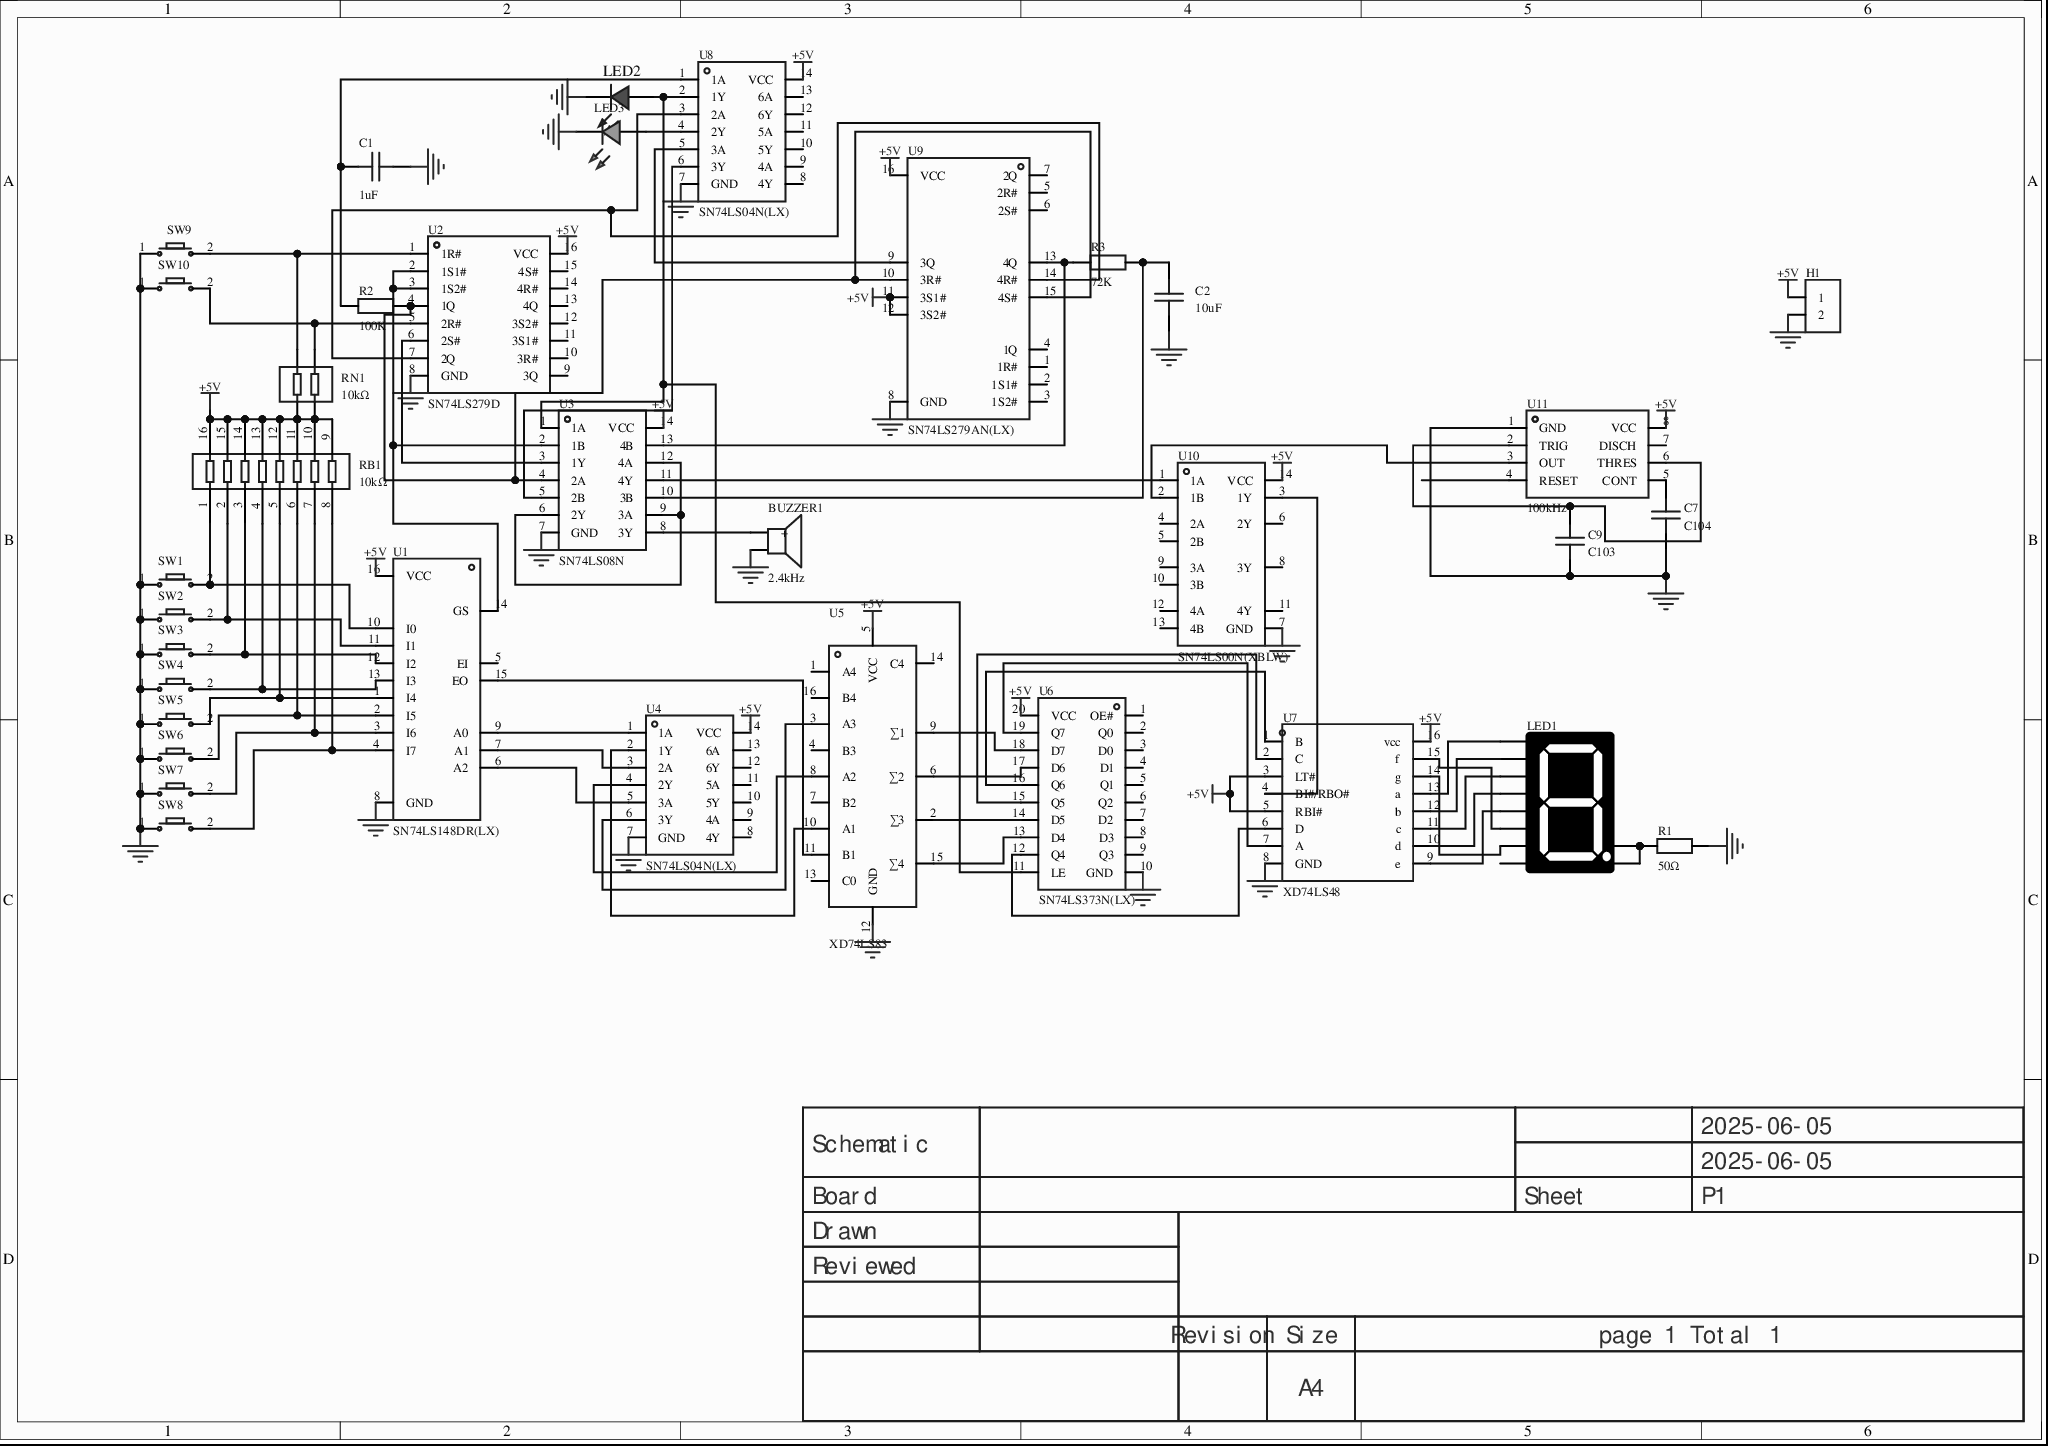
[diagram p0: MISC51700-3.schdoc]
# Altium project MISC51700-2.PrjPcb
1 sheet, 35 parts. Net scope: global (net labels, ports and power ports of the same name join across sheets).
Board file: MISC51700.pcbdoc

## Sheet MISC51700-3.schdoc
size 297 x 209 mm; Version: V1.0; @Project Name: MISC51700; @Page Count: 1; @Update Date: 2025-06-05; @Create Date: 2025-06-05; @Schematic Name: MISC51700; @Page No: 1; @Create Time: 06:48:36; @Update Time: 17:09:20; @Board Name: MISC51700

### Parts
BUZZER1  2.4kHz  [BUZ-TH_BD12.0-P7.60-D0.6-FD]
C1  1uF  [C0603]
C2  10uF  [C0603]
C7  C104  [CAP-TH_L8.5-W5.0-P5.00-D1.2]
C9  C103  [CAP-TH_L8.5-W5.0-P5.00-D1.2]
H1  (no value)  [HDR-TH_2P-P2.54-V-F]
LED1  (no value)  [LED-SEG-TH_10P-L12.6-W19.0-P2.54-S15.24-BL]
LED2  (no value)  [LED_0805]
LED3  (no value)  [LED_0805]
R1  50Ω  [R0603]
R2  100K  [R0805]
R3  72K  [R0805]
RB1  10kΩ  [RES-ARRAY-SMD_0603-16P-L6.4-W1.6-TL]
RN1  10kΩ  [RES-ARRAY-SMD_0603-4P-L1.6-W1.6-BL]
SW1  (no value)  [Key_SMD_3x4x2]
SW2  (no value)  [Key_SMD_3x4x2]
SW3  (no value)  [Key_SMD_3x4x2]
SW4  (no value)  [Key_SMD_3x4x2]
SW5  (no value)  [Key_SMD_3x4x2]
SW6  (no value)  [Key_SMD_3x4x2]
SW7  (no value)  [Key_SMD_3x4x2]
SW8  (no value)  [Key_SMD_3x4x2]
SW9  (no value)  [Key_SMD_3x4x2]
SW10  (no value)  [Key_SMD_3x4x2]
U1  SN74LS148DR(LX)  [SOIC-16_L9.9-W3.9-P1.27-LS6.0-BL-1]
U2  SN74LS279D  [SOIC-16_L9.9-W3.9-P1.27-LS6.0-BL]
U3  SN74LS08N  [PDIP-14_L19.3-W6.4-P2.54-LS7.9-BL-1]
U4  SN74LS04N(LX)  [DIP-14_L19.1-W6.4-P2.54-LS7.6-BL]
U5  XD74LS83  [PDIP-16_L19.1-W6.4-P2.54-LS7.62-BL]
U6  SN74LS373N(LX)  [PDIP-20_L26.2-W7.6-P2.54-LS7.9-BL]
U7  XD74LS48  [DIP-16_L19.3-W6.4-P2.54-LS7.6-BL]
U8  SN74LS04N(LX)  [DIP-14_L19.1-W6.4-P2.54-LS7.6-BL]
U9  SN74LS279AN(LX)  [PDIP-16_L19.3-W6.4-P2.54-LS7.94-BL]
U10  SN74LS00N(XBLW)  [PDIP-14_L19.3-W6.4-P2.54-LS7.6-BL]
U11  100kHz  [DIP-8_L9.8-W6.6-P2.54-LS7.6-BL]

### Nets
+5V: H1.1 RB1.9 RB1.10 RB1.11 RB1.12 RB1.13 RB1.14 RB1.15 RB1.16 RN1.1 RN1.2 U1.16(VCC) U2.16(VCC) U3.14(VCC) U4.14(VCC) U5.5(VCC) U6.20(VCC) U7.3(LT#) U7.5(RBI#) U7.16(vcc) U8.14(VCC) U9.11(3S1#) U9.12(3S2#) U9.16(VCC) U10.14(VCC) U11.8(VCC)
GND: BUZZER1.2 C1.2 C2.1 C7.1 C9.1 H1.2 LED2.1(C) LED3.1(C) R1.1 SW1.1 SW2.1 SW3.1 SW4.1 SW5.1 SW6.1 SW7.1 SW8.1 SW9.1 SW10.1 U1.8(GND) U2.8(GND) U3.7(GND) U4.7(GND) U5.12(GND) U6.10(GND) U7.8(GND) U8.7(GND) U9.8(GND) U10.7(GND) U11.1(GND)
NetBUZZER1_1: BUZZER1.1(+) U3.8(3Y)
NetC1_1: C1.1 R2.1 U8.1(1A)
NetC2_2: C2.2 R3.2 U3.10(3B)
NetC7_2: C7.2 U11.5(CONT)
NetC9_2: C9.2 U11.2(TRIG) U11.6(THRES)
NetLED1_1: LED1.1(E) U7.9(e)
NetLED1_2: LED1.2(D) U7.10(d)
NetLED1_3: LED1.3(G1) LED1.8(G2) R1.2
NetLED1_4: LED1.4(C) U7.11(c)
NetLED1_6: LED1.6(B) U7.12(b)
NetLED1_7: LED1.7(A) U7.13(a)
NetLED1_9: LED1.9(F) U7.15(f)
NetLED1_10: LED1.10(G) U7.14(g)
NetLED2_2: LED2.2(A) U3.1(1A) U6.11(LE) U8.2(1Y)
NetLED3_2: LED3.2(A) U8.4(2Y)
NetR2_2: R2.2 U2.4(1Q) U3.4(2A) U9.10(3R#) U9.15(4S#)
NetR3_1: R3.1 U3.13(4B) U9.13(4Q)
NetRB1_1: RB1.1 SW1.2 U1.10(I0)
NetRB1_2: RB1.2 SW2.2 U1.11(I1)
NetRB1_3: RB1.3 SW3.2 U1.12(I2)
NetRB1_4: RB1.4 SW4.2 U1.13(I3)
NetRB1_5: RB1.5 SW5.2 U1.1(I4)
NetRB1_6: RB1.6 SW6.2 U1.2(I5)
NetRB1_7: RB1.7 SW7.2 U1.3(I6)
NetRB1_8: RB1.8 SW8.2 U1.4(I7)
NetRN1_3: RN1.3 SW10.2 U2.5(2R#)
NetRN1_4: RN1.4 SW9.2 U2.1(1R#)
NetU1_6: U1.6(A2) U4.5(3A)
NetU1_7: U1.7(A1) U4.3(2A)
NetU1_9: U1.9(A0) U4.1(1A)
NetU1_14: U1.14(GS) U2.2(1S1#) U2.3(1S2#) U3.2(1B)
NetU1_15: U1.15(EO) U5.11(B1)
NetU2_6: U2.6(2S#) U3.3(1Y)
NetU2_7: U2.7(2Q) U8.3(2A) U9.14(4R#)
NetU3_5: U3.5(2B) U8.6(3Y)
NetU3_6: U3.6(2Y) U3.9(3A) U3.12(4A)
NetU3_11: U3.11(4Y) U10.1(1A)
NetU4_2: U4.2(1Y) U5.10(A1)
NetU4_4: U4.4(2Y) U5.8(A2)
NetU4_6: U4.6(3Y) U5.3(A3)
NetU5_2: U5.2(∑3) U6.14(D5)
NetU5_6: U5.6(∑2) U6.17(D6)
NetU5_9: U5.9(∑1) U6.18(D7)
NetU5_15: U5.15(∑4) U6.13(D4)
NetU6_12: U6.12(Q4) U7.6(D)
NetU6_15: U6.15(Q5) U7.2(C)
NetU6_16: U6.16(Q6) U7.1(B)
NetU6_19: U6.19(Q7) U7.7(A)
NetU7_4: U7.4(BI#/RBO#) U10.3(1Y)
NetU8_5: U8.5(3A) U9.9(3Q)
NetU10_2: U10.2(1B) U11.3(OUT)

Not connected (* = marked no-connect by the designer): LED1 5(DP); U1 5(EI); U2 9(3Q) 10(3R#) 11(3S1#) 12(3S2#) 13(4Q) 14(4R#) 15(4S#); U4 8(4Y) 9(4A) 10(5Y) 11(5A) 12(6Y) 13(6A); U5 1(A4) 4(B3) 7(B2) 13(C0) 14(C4) 16(B4); U6 1(OE#) 2(Q0) 3(D0) 4(D1) 5(Q1) 6(Q2) 7(D2) 8(D3) 9(Q3); U8 8(4Y) 9(4A) 10(5Y) 11(5A) 12(6Y) 13(6A); U9 1(1R#) 2(1S1#) 3(1S2#) 4(1Q) 5(2R#) 6(2S#) 7(2Q); U10 4(2A) 5(2B) 6(2Y) 8(3Y) 9(3A) 10(3B) 11(4Y) 12(4A) 13(4B); U11 4(RESET) 7(DISCH)

### Notes on the sheet
- 2025-06-05
- Schematic
- Board
- Sheet
- P1
- Drawn
- Reviewed
- Revision
- Size
- A4
- page 1 Total 1

### Library data of the parts
BUZZER1 = TMB12A05_C96093: Drive mode:Active (built-in driver); Construction:Electromagnetic; Rated voltage:-; Frequency:2.4kHz; Sound pressure (SPL):85dB;; Manufacturer: 华能; AddInBom: yes; ModelId: 16ab50e14c5b4f2c986c135bdba60e37; ModelName: BUZ-TH_D12.0-H9.5-P7.60; ModelTransform: 472.44,472.176,0,90,0,0,-0.787,0,-177.165; Voltage - Supply: 4V~8V; Sound Pressure Level(SPL): 85dB; Symbol: TMB12A05; Device: TMB12A05_C96093; LCSC Part Name: TMB12A05; SupplierPart: C96093; ManufacturerPart: TMB12A05; Supplier Footprint: 插件,D=12mm; JLCPCB Part Class: Extended library; Datasheet: https://example.com/upload/public/pdf/source/20241025/8A17FE04D767D19A35A06DEF9A82AB1E.pdf; Supplier: LCSC; ConvertToPcb: yes; FootprintName: BUZ-TH_BD12.0-P7.60-D0.6-FD; Driver Circuitry: Active (built-in driver); Technology: Electromagnetic; Voltage Rating: -; Value: 2.4kHz; Current Consumption: -; Diameter(φD): 12mm; Length: -; Width: -; Height: 9.8mm; Operating Temperature: -
C1 C2 = CAP_0603: ConvertToPcb: yes; SymbolName: CapAcitance; ModelId: ac125912035d415993ca9572d50418b1; ModelName: C0603_L1.6-W0.8-H0.8; ModelTransform: 62.992,31.496,0,0,0,0,0,0,0; Device: CAP_0603; AddInBom: yes; Supplier Footprint: 0603; FootprintName: C0603
  C1: Value: 1uF
  C2: Value: 10uF
C7 C9 = CT4-0805B104K500F3: Capacitance:100nF; Tolerance:±10%; Rated voltage:50V; Temp coefficient:X7R;; Manufacturer: FH(风华); AddInBom: yes; ModelId: 5610b656e7164072960d9d2d8c7d4fdf; ModelName: CAP-TH_L4.2-W3.8-H3.8-P5.08; ModelTransform: 222.8342,149.606,0,0,0,0,0,0,-118.11; Tolerance: ±10%; Voltage Rated: 50V; Temperature Coefficient: X7R; Symbol: CT4-0805B104K500F3; Device: CT4-0805B104K500F3; LCSC Part Name: 100nF ±10% 50V C3型（直脚）; ManufacturerPart: CT4-0805B104K500F3; Supplier Footprint: 插件,P=5.08mm; JLCPCB Part Class: Extended library; Datasheet: https://example.com/upload/public/pdf/source/20190402/C385200_059806A6312B28FF1421A2413EB641E1.pdf; Supplier: LCSC; ConvertToPcb: yes; FootprintName: CAP-TH_L8.5-W5.0-P5.00-D1.2
  C7: Value: C104
  C9: Value: C103
H1 = HDR-F_2.54_1x2P: Symbol: Header-Female-2.54_1x2; ConvertToPcb: yes; ModelId: a9450ef445564560a104363b9aacde4e; ModelName: HDR-TH_2P-P2.54-F-LI-1X2P; ModelTransform: 215.7476,98.425,0,0,0,0,0,0,-129.921; Device: HDR-F_2.54_1x2P; AddInBom: yes; SupplierPart: C49661; Supplier Footprint: 插件; FootprintName: HDR-TH_2P-P2.54-V-F
LED1 = LED_SEG_TH_0.56x1: Symbol: LED_SEG_TH_0.56*1; ConvertToPcb: yes; ModelId: 16c3aae6d39e4ecc9e744d6eeac8d57b; ModelName: LED-SEG-TH_0.56_1p; ModelTransform: 496.062,748.03,0,0,0,0,0,0,-137.795; Device: LED_SEG_TH_0.56x1; AddInBom: yes; Supplier Footprint: 插件; FootprintName: LED-SEG-TH_10P-L12.6-W19.0-P2.54-S15.24-BL
LED2 = LED_0805-R: Symbol: LED_R; Convert to PCB: yes; 3D Model: 33fb9fca58e84f37a403ebeef4c28b77; 3D Model Transform: 78.7,49.1,39.3,0,0,0,0,0,0; ModelName: LED-0805_R; Device: LED_0805-R; Add into BOM: yes; Supplier Footprint: 0805; FootprintName: LED_0805
LED3 = LED_0805-G: Symbol: LED_G; Convert to PCB: yes; 3D Model: 381ae4d721d6485eaad9d0ca067812b5; 3D Model Transform: 63.9,39.8,31.9,0,0,0,0,0,0; ModelName: LED-0805_G; Device: LED_0805-G; Add into BOM: yes; Supplier Footprint: 0805; FootprintName: LED_0805
R1 = Res_0603: ConvertToPcb: yes; SymbolName: Resistor; ModelId: fc143cca1e79419f9cd78b61e9279f08; ModelTransform: 31.8897,63.7794,0,90,0,0,0,0,0; Value: 50Ω; Device: Res_0603; AddInBom: yes; Supplier Footprint: 0603; FootprintName: R0603; ModelName: R0603
R2 R3 = Res_0805: ConvertToPcb: yes; SymbolName: Resistor; ModelId: 37a81e68749a4138bd2dfa6897b24b85; ModelName: R0805_L2.0-W1.3-H0.6; ModelTransform: 78.74,51.181,0,0,0,0,0,-0.0005,0; Device: Res_0805; AddInBom: yes; Supplier Footprint: 0805; FootprintName: R0805
  R2: Value: 100K
  R3: Value: 72K
RB1 = 742C163103JP: Resistor count:8; Resistance:10kΩ; Tolerance:±5%; Power per element:63mW; Temp coefficient:±200ppm/℃;; Manufacturer: CTS(西迪斯); AddInBom: yes; ModelId: 221f6fb4f2034148a9d47d497d859194; ModelTransform: 251.968,64.961,0,0,0,0,0,0,0; Number of Resistors: 8; Tolerance: ±5%; Power(Watts): 63mW; Symbol: 742C163103JP; Device: 742C163103JP; LCSC Part Name: 10kΩ ±5%; SupplierPart: C2654035; ManufacturerPart: 742C163103JP; Supplier Footprint: 0603x8; JLCPCB Part Class: Extended library; Datasheet: https://example.com/upload/public/pdf/source/20210503/EA698ADAEE513162139F7667D383C0D0.pdf; Supplier: LCSC; ConvertToPcb: yes; FootprintName: RES-ARRAY-SMD_0603-16P-L6.4-W1.6-TL; ModelName: RES-ARRAY-SMD_0603-16P-L6.4-W1.6-TL; Value: 10kΩ; Temperature Coefficient: ±200ppm/℃; Number of Pins: 16
RN1 = 2D03WGJ0103T5E: Resistor count:2; Resistance:10kΩ; Tolerance:±5%; Power per element:62.5mW; Temp coefficient:±200ppm/℃;; Manufacturer: UNI-ROYAL(厚声); AddInBom: yes; ModelId: c28f3269927844d1bae4b585f2f82e94; ModelName: RES-ARRAY-SMD_0603-4P-L1.6-W1.6-H0.5-BL; ModelTransform: 62.992,62.992,0,0,0,0,0,0,0; Number of Resistors: 2; Tolerance: ±5%; Power(Watts): 62.5mW; Symbol: 2D03WGJ0103T5E; Device: 2D03WGJ0103T5E; LCSC Part Name: 10kΩ ±5%; SupplierPart: C2765531; ManufacturerPart: 2D03WGJ0103T5E; Supplier Footprint: 0603x2; JLCPCB Part Class: Extended library; Datasheet: https://example.com/upload/public/pdf/source/20210330/C2758625_90D19EEA9B8C23AA9BAF71D52BD1DB3E.pdf; Supplier: LCSC; ConvertToPcb: yes; FootprintName: RES-ARRAY-SMD_0603-4P-L1.6-W1.6-BL; Value: 10kΩ; Temperature Coefficient: ±200ppm/℃; Number of Pins: 4
SW1-SW10 = Key_SMD_3x4x2: ConvertToPcb: yes; SymbolName: Tactile switch x2; ModelId: 63599cce708d48afbce1b0db003544770819f05c4eef4c71ace90d822a990e87; ModelName: SW-SMD_L4.0-W2.9-H2-LS5.0; ModelTransform: 196.85,114.17,79.13,0,0,0,0,0,0; Device: Key_SMD_3x4x2; AddInBom: yes; Supplier Footprint: SMD; FootprintName: Key_SMD_3x4x2
U1 = SN74LS148DR(LX): Manufacturer: LX(灵星芯微); AddInBom: yes; ModelId: 19d62df4453549be81db7b702f301941; ModelName: SOIC-16_L9.9-W3.9-H1.8-LS6.0-P1.27; ModelTransform: 389.763,236.454,0,0,0,0,0,0,0; Symbol: SN74LS148DR(LX); Device: SN74LS148DR(LX); LCSC Part Name: SN74LS148DR(LX); SupplierPart: C32710673; ManufacturerPart: SN74LS148DR(LX); Supplier Footprint: SOP-16; JLCPCB Part Class: Extended library; Datasheet: https://example.com/upload/public/pdf/source/20240417/102B6FDCFA309F0B30F1058715E63CF7.pdf; Supplier: LCSC; ConvertToPcb: yes; FootprintName: SOIC-16_L9.9-W3.9-P1.27-LS6.0-BL-1
U2 = SN74LS279D: Manufacturer: onsemi(安森美); AddInBom: yes; ModelId: c21ec766ec2643efb3352f8441994f4e; ModelName: SOIC-16_L9.9-W3.9-H1.8-LS6.0-P1.27; ModelTransform: 389.763,236.454,0,0,0,0,0,0,0; Symbol: SN74LS279D; Device: SN74LS279D; LCSC Part Name: SN74LS279D; SupplierPart: C3826626; ManufacturerPart: SN74LS279D; Supplier Footprint: -; JLCPCB Part Class: Extended library; Datasheet: https://example.com/upload/public/pdf/source/20230915/97FED84B533BE8D9150AD31DF08D2AAB.pdf; Supplier: LCSC; ConvertToPcb: yes; FootprintName: SOIC-16_L9.9-W3.9-P1.27-LS6.0-BL
U3 = SN74LS08N: Logic type:AND gate; Channels:4; Operating voltage:4.75V~5.25V; Propagation delay (tpd):-;; Manufacturer: TI(德州仪器); AddInBom: yes; ModelId: 850da569defe42bfb44bffbf61585822; ModelTransform: 751.967,309.842,0,0,0,0,0,0,-118.11; Number of Channels: 4; Current - Output Low(IOL): 8mA; Current - Output High(IOH): 400uA; Input Logic Level - High: 2V; Input Logic Level - Low: 800mV; Symbol: SN74LS08N; Device: SN74LS08N; LCSC Part Name: SN74LS08N; SupplierPart: C2869595; ManufacturerPart: SN74LS08N; Supplier Footprint: PDIP-14; JLCPCB Part Class: Extended library; Supplier: LCSC; ConvertToPcb: yes; FootprintName: PDIP-14_L19.3-W6.4-P2.54-LS7.9-BL-1; ModelName: PDIP-14_L19.3-W6.4-P2.54-LS7.9-BL-1; Logic Type: AND gate; Voltage - Supply: 4.75V~5.25V; Series: 74LS series; Propagation Delay: -; Operating Temperature: 0℃~+70℃
U4 U8 = SN74LS04N(LX): Operating voltage:2V~6V; Operating current:2uA; Channels:6; Propagation delay (tpd):14ns@6V;; Manufacturer: LX(灵星芯微); AddInBom: yes; ModelId: 4fb82330961949e587245d1f3ebad69c; ModelTransform: 751.967,324.8025,0,0,0,0,0,0,-118.11; Voltage - Supply: 2V~6V; Current - Supply: 2uA; Number of Circuits: 6; Current - Output Low(IOL): 5.2mA; Input Logic Level - High: 1.5V~4.2V; Input Logic Level -Low: 500mV~1.8V; Output Logic Level - Low: 100mV~260mV; Symbol: SN74LS04N(LX); Device: SN74LS04N(LX); LCSC Part Name: SN74LS04N(LX); SupplierPart: C22374093; ManufacturerPart: SN74LS04N(LX); Supplier Footprint: DIP-14; JLCPCB Part Class: Extended library; Datasheet: https://example.com/upload/public/pdf/source/20240402/834FB3A59B1B710673385084ADD2A13F.pdf; Supplier: LCSC; ConvertToPcb: yes; FootprintName: DIP-14_L19.1-W6.4-P2.54-LS7.6-BL; ModelName: DIP-14_L19.1-W6.4-P2.54-LS7.6-BL; Current - Output High(IOH): 5.2mA; Output Logic Level - High: -; Max Propagation Delay: 14ns@6V; Series: 74LS series; Operating Temperature: -40℃~+125℃
U5 = XD74LS83: Channels:2; Operating voltage:5V;; Manufacturer: XINLUDA(信路达); AddInBom: yes; ModelId: ee2b051935954f8aa1bc820113d1de81; ModelTransform: 749.99858,309.842,0,0,0,0,0,0,-196.85; Logic Type: Full adder with fast carry; Number of Channels: 2; Voltage - Supply: 5V; Symbol: XD74LS83; Device: XD74LS83; LCSC Part Name: XD74LS83; SupplierPart: C968685; ManufacturerPart: XD74LS83; Supplier Footprint: DIP-16; JLCPCB Part Class: Extended library; Datasheet: https://example.com/upload/public/pdf/source/20241011/6F4CFFC09F59AEBAD3597393677468D3.pdf; Supplier: LCSC; ConvertToPcb: yes; FootprintName: PDIP-16_L19.1-W6.4-P2.54-LS7.62-BL; ModelName: PDIP-16_L19.1-W6.4-P2.54-LS7.62-BL; Operating Temperature: 0℃~+70℃
U6 = SN74LS373N(LX): Logic type:D-type latch; Operating voltage:2V~6V; Channels:8; Propagation delay (tpd):26ns;; Manufacturer: LX(灵星芯微); AddInBom: yes; ModelId: 872b430e9c8d40c7a02b132014944e6a; ModelTransform: 1031.494,309.842,0,0,0,0,0,0,-149.606; Output Type: Tri-state; Voltage - Supply: 2V~6V; Number of Channels: 8; Current - Output High(IOH): 7.8mA; Propagation Delay Time: 26ns; Symbol: SN74LS373N(LX); Device: SN74LS373N(LX); LCSC Part Name: SN74LS373N(LX); SupplierPart: C22374106; ManufacturerPart: SN74LS373N(LX); Supplier Footprint: DIP-20; JLCPCB Part Class: Extended library; Datasheet: https://example.com/upload/public/pdf/source/20240402/EFE2DAB80863AAE41F14BDA3484332FE.pdf; Supplier: LCSC; ConvertToPcb: yes; FootprintName: PDIP-20_L26.2-W7.6-P2.54-LS7.9-BL; ModelName: PDIP-20_L26.2-W7.6-P2.54-LS7.9-BL; Logic Type: D-type latch; Current - Output Low(IOL): 7.8mA; Series: 74LS; Operating Temperature: -40℃~+125℃
U7 = XD74LS48: Decoder/driver, 4-to-7; Manufacturer: XINLUDA(信路达); AddInBom: yes; ModelId: 6a0b9f170db542aa9e288f652469859c; ModelTransform: 759.841,309.842,0,0,0,0,0,0,-118.11; Symbol: XD74LS48; Device: XD74LS48; LCSC Part Name: XD74LS48; SupplierPart: C609759; ManufacturerPart: XD74LS48; Supplier Footprint: DIP-16; JLCPCB Part Class: Extended library; Datasheet: https://example.com/upload/public/pdf/source/20240625/ADBA044A35F7C4DB2F31130498A5586F.pdf; Supplier: LCSC; ConvertToPcb: yes; FootprintName: DIP-16_L19.3-W6.4-P2.54-LS7.6-BL; ModelName: DIP-16_L19.3-W6.4-P2.54-LS7.6-BL
U9 = SN74LS279AN(LX): Logic type:S-R latch; Supply voltage:2V~6V; Channels:4; Propagation delay:33ns;; Manufacturer: LX(灵星芯微); AddInBom: yes; ModelId: 96ff5d01b3074dd183bcbc4cd00a63de; ModelTransform: 759.841,322.44,0,0,0,0,0,0,-137.795; Supply Voltage: 2V~6V; Number of Channels: 4; Propagation Delay: 33ns; Symbol: SN74LS279AN(LX); Device: SN74LS279AN(LX); LCSC Part Name: SN74LS279AN(LX); SupplierPart: C41430933; ManufacturerPart: SN74LS279AN(LX); Supplier Footprint: DIP-16; JLCPCB Part Class: Extended library; Datasheet: https://example.com/upload/public/pdf/source/20241015/677F81D993056D0E07AF30CD46A3A6BE.pdf; Supplier: LCSC; ConvertToPcb: yes; FootprintName: PDIP-16_L19.3-W6.4-P2.54-LS7.94-BL; ModelName: PDIP-16_L19.3-W6.4-P2.54-LS7.94-BL; Logic Type: S-R latch; Output Type: -; Source Current: -; Sink Current: -; Series: -; OperatingTemperature: -40℃~+125℃
U10 = SN74LS00N(XBLW): SN74LS00 is a quad 2-input NAND gate; inputs include clamp diodes, allowing a current-limiting resistor to connect the input to a voltage above Vcc.; Manufacturer: XBLW(芯伯乐); AddInBom: yes; ModelId: ca4ed987146b49a5a2d3ca847d6466c4; ModelTransform: 755.904,309.842,0,0,0,0,0,0,-125.984; Symbol: SN74LS00N(XBLW); Device: SN74LS00N(XBLW); LCSC Part Name: SN74LS00N(XBLW); SupplierPart: C42395504; ManufacturerPart: SN74LS00N(XBLW); Supplier Footprint: DIP-14; JLCPCB Part Class: Extended library; Datasheet: https://example.com/upload/public/pdf/source/20241125/0067A7F7C2DEF0E0B5DA6BC8FA4D490C.pdf; Supplier: LCSC; ConvertToPcb: yes; FootprintName: PDIP-14_L19.3-W6.4-P2.54-LS7.6-BL; ModelName: PDIP-14_L19.3-W6.4-P2.54-LS7.6-BL
U11 = NE555P: Frequency:100kHz;; Manufacturer: TI(德州仪器); AddInBom: yes; ModelId: db2af726fcec488f8bf8e467aca974b3; ModelName: DIP-8_L9.8-W6.6-H3.5-LS7.62-P2.54; ModelTransform: 385.826,311.8104,0,0,0,0,-1.693,0,-137.795; Supply Voltage: 4.5V~16V; Supply Current: 10mA; Symbol: NE555P; Device: NE555P; LCSC Part Name: NE555P; SupplierPart: C46749; ManufacturerPart: NE555P; Supplier Footprint: DIP-8; JLCPCB Part Class: Extended library; Supplier: LCSC; ConvertToPcb: yes; FootprintName: DIP-8_L9.8-W6.6-P2.54-LS7.6-BL; Value: 100kHz; Operating Temperature: 0℃~+70℃